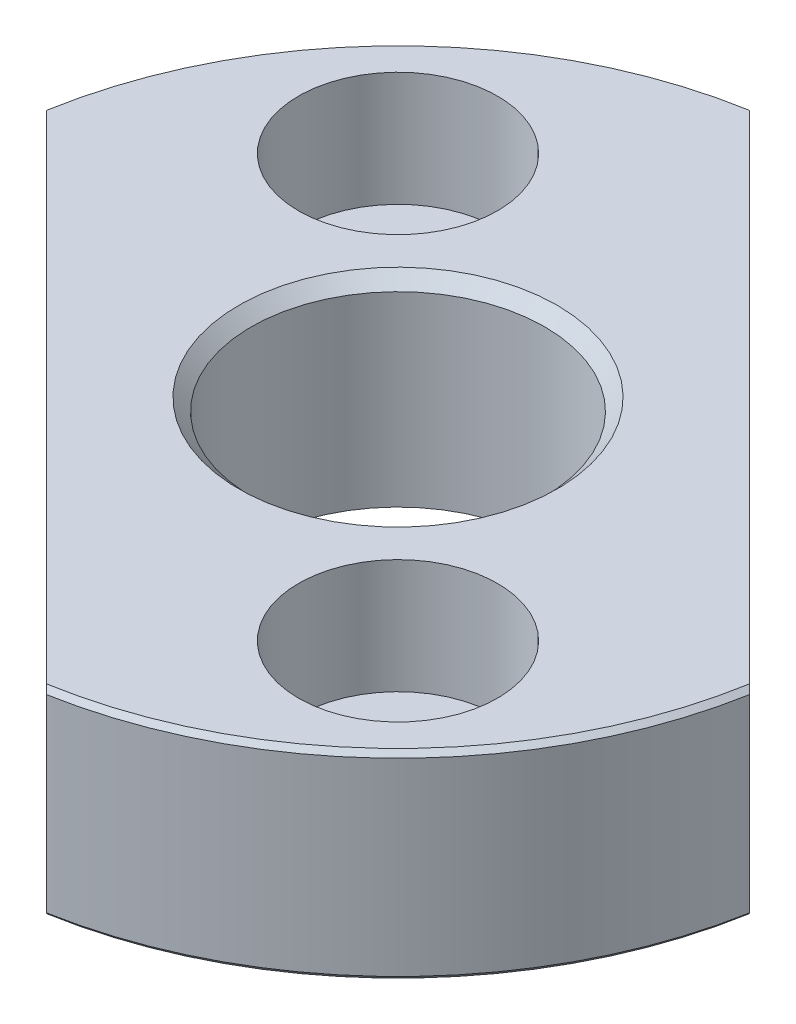
from build123d import *

# Parameters (mm, degrees)
G1_4_TAPPED_HOLE1_D                               = 11.8
HOLE_SIZE_BASED_ON_SOCKET_HEAD_CAP_SC_D           = 4.8
HOLE_SIZE_BASED_ON_SOCKET_HEAD_CAP_SC_CBORE_D     = 8
HOLE_SIZE_BASED_ON_SOCKET_HEAD_CAP_SC_CBORE_DEPTH = 4.6
FILLET1_R                                         = 0.2
CHAMFER1_SIZE                                     = 0.2
CHAMFER2_SIZE                                     = 0.5
CUT_EXTRUDE1_DEPTH                                = 35.474628352
SKETCH8_R                                         = 15
CUT_EXTRUDE2_DEPTH                                = 30.145808143


with BuildPart() as part:
    # Sketch2 → Revolve1 (revolve)
    with BuildSketch(Plane.XY, mode=Mode.PRIVATE) as revolve1_sk:
        Polygon((0, 24), (-17.5, 24), (-17.5, 16), (-6.75, 16), (-6.75, 0), (0, 0), align=None)
    revolve(revolve1_sk.sketch.rotate(Axis((0, 0, 0), (0, 1, 0)), 270), axis=Axis((0, 0, 0), (0, 1, 0)))

    # G1/4 Tapped Hole1 (through all)
    with Locations(Plane.ZX.offset(24)):
        with Locations((0, 0)):
            Hole(G1_4_TAPPED_HOLE1_D / 2)

    # Hole Size (% based on) Socket Head Cap Screw Type 1 (through all)
    with Locations(Plane(origin=(-8.485281374, 24, -8.485281374), x_dir=(0, 0, 1), z_dir=(0, 1, 0))):
        with Locations((0, 0), (16.970562748, 16.970562748)):
            CounterBoreHole(HOLE_SIZE_BASED_ON_SOCKET_HEAD_CAP_SC_D / 2, HOLE_SIZE_BASED_ON_SOCKET_HEAD_CAP_SC_CBORE_D / 2, HOLE_SIZE_BASED_ON_SOCKET_HEAD_CAP_SC_CBORE_DEPTH)

    # Fillet1
    fillet1_edges = [part.edges().sort_by_distance(p)[0] for p in [
        (0, 16, 6.75),
    ]]
    fillet(fillet1_edges, radius=FILLET1_R)

    # Chamfer1
    chamfer1_edges = [part.edges().sort_by_distance(p)[0] for p in [
        (0, 0, 6.75),
        (0, 16, 17.5),
        (0, 24, 17.5),
    ]]
    chamfer(chamfer1_edges, length=CHAMFER1_SIZE)

    # Chamfer2
    chamfer2_edges = [part.edges().sort_by_distance(p)[0] for p in [
        (0, 24, 5.9),
        (0, 0, 5.9),
    ]]
    chamfer(chamfer2_edges, length=CHAMFER2_SIZE)

    # Sketch7 → Cut-Extrude1 (cut, through all)
    with BuildSketch(Plane(origin=(0, 24, 0), x_dir=(1, 0, 0), z_dir=(0, 1, 0))):
        with BuildLine():
            Line((2.911166407, -17.053302031), (-17.053302031, 2.911166407))
            ThreePointArc((-17.053302031, 2.911166407), (-12.232947315, -12.232947315), (2.911166407, -17.053302031))
        make_face()
        with BuildLine():
            ThreePointArc((17.3, 0), (11.156317071, 13.222200627), (-2.911166407, 17.053302031))
            Line((-2.911166407, 17.053302031), (17.053302031, -2.911166407))
            ThreePointArc((17.053302031, -2.911166407), (17.238215179, -1.460800272), (17.3, 0))
        make_face()
        with BuildLine():
            Line((-17.053302031, 2.911166407), (-17.226115818, 3.083980194))
            ThreePointArc((-17.226115818, 3.083980194), (-12.374368671, -12.374368671), (3.083980194, -17.226115818))
            Line((3.083980194, -17.226115818), (2.911166407, -17.053302031))
            ThreePointArc((2.911166407, -17.053302031), (-12.232947315, -12.232947315), (-17.053302031, 2.911166407))
        make_face()
        with BuildLine():
            ThreePointArc((17.5, 0), (11.23121424, 13.42050024), (-3.083980194, 17.226115818))
            Line((-3.083980194, 17.226115818), (-2.911166407, 17.053302031))
            ThreePointArc((-2.911166407, 17.053302031), (11.156317071, 13.222200627), (17.3, 0))
            ThreePointArc((17.3, 0), (17.238215179, -1.460800272), (17.053302031, -2.911166407))
            Line((17.053302031, -2.911166407), (17.226115818, -3.083980194))
            ThreePointArc((17.226115818, -3.083980194), (17.431394477, -1.548058977), (17.5, 0))
        make_face()
    extrude(amount=-CUT_EXTRUDE1_DEPTH, mode=Mode.SUBTRACT)

    # Sketch8 → Cut-Extrude2 (cut, through all)
    with BuildSketch(Plane.XZ.offset(-16)):
        Circle(SKETCH8_R)
    extrude(amount=CUT_EXTRUDE2_DEPTH, mode=Mode.SUBTRACT)


solid = part.part
